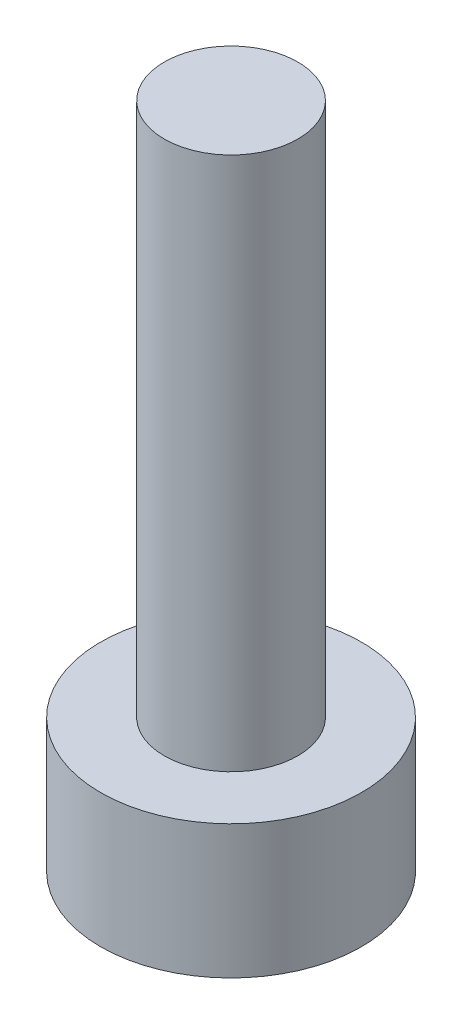
SolidWorks part; units mm, degrees
ref_plane "Front Plane" through (0, 0, 0) normal (0, 0, 1) x (1, 0, 0)
ref_plane "Top Plane" through (0, 0, 0) normal (0, 1, 0) x (1, 0, 0)
ref_plane "Right Plane" through (0, 0, 0) normal (1, 0, 0) x (0, 0, -1)
sketch "Sketch2" plane through (0, 0, 0) normal (0, 1, 0) x (1, 0, 0)
  circle A0 centre (0, 0) radius 2.93
extrude "Boss-Extrude1" add sketch "Sketch2" along normal blind 3
sketch "Sketch3" plane through (0, 3, 0) normal (0, 1, 0) x (1, 0, 0)
  circle A0 centre (0, 0) radius 1.5
extrude "Boss-Extrude2" add sketch "Sketch3" along normal blind 12
cosmetic thread "Cosmetic Thread1" parameters "D1"=6, "D2"=2.459
sketch "Sketch4" plane through (0, 0, 0) normal (0, -1, 0) x (1, 0, 0)
  line L1 (0.9898, 0.8273) -> (-0.2216, 1.2708)
  line L2 (-0.2216, 1.2708) -> (-1.2114, 0.4435)
  line L3 (-1.2114, 0.4435) -> (-0.9898, -0.8273)
  line L4 (-0.9898, -0.8273) -> (0.2216, -1.2708)
  line L5 (0.2216, -1.2708) -> (1.2114, -0.4435)
  line L6 (1.2114, -0.4435) -> (0.9898, 0.8273)
  circle A0 centre (0, 0) radius 1.29 construction
extrude "Cut-Extrude1" cut sketch "Sketch4" against normal blind 1.3
